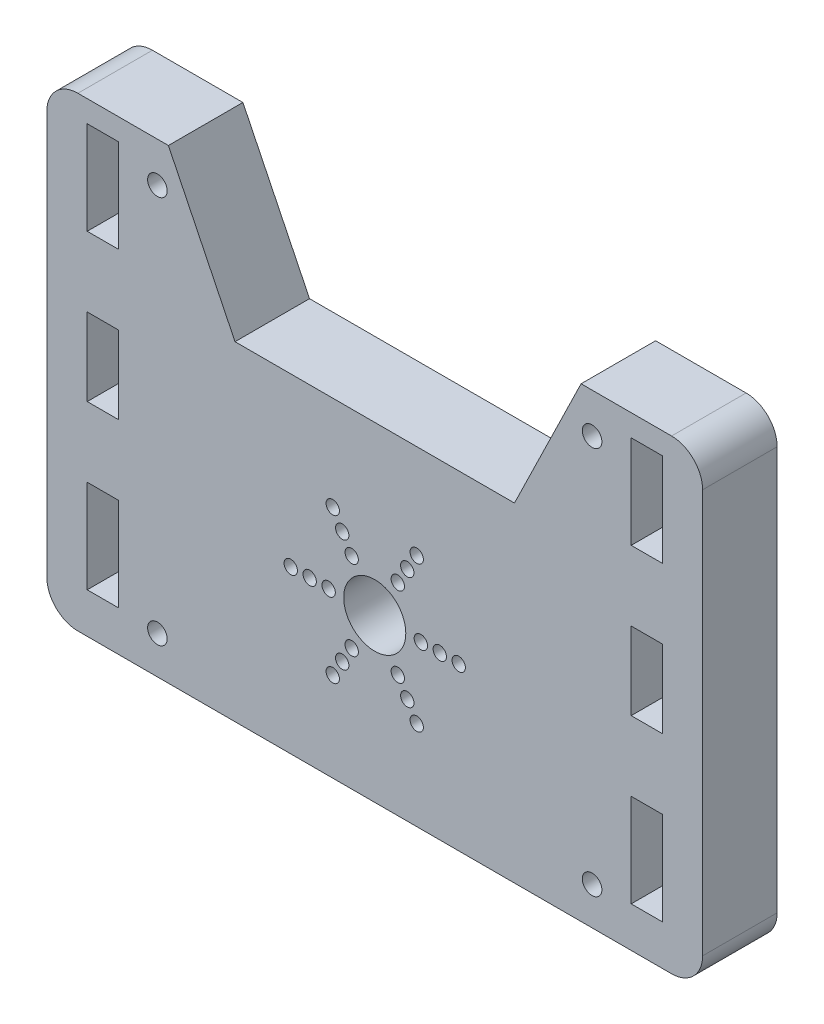
SolidWorks part; units mm, degrees
ref_plane "前视基准面" through (0, 0, 0) normal (0, 0, 1) x (1, 0, 0)
ref_plane "上视基准面" through (0, 0, 0) normal (0, 1, 0) x (1, 0, 0)
ref_plane "右视基准面" through (0, 0, 0) normal (1, 0, 0) x (0, 0, -1)
other "Configuration Table"
sketch "草图1" plane through (0, 0, 0) normal (0, 0, 1) x (1, 0, 0)
  line L0 (0, 52.9649) -> (0, -55.4114) construction
  line L1 (-89.1236, 0) -> (105.0799, 0) construction
  line L2 (-33.1441, 37.4747) -> (-22.414, 15.4747)
  line L3 (-47.714, 37.4747) -> (-33.1441, 37.4747)
  line L4 (-52.714, 32.4747) -> (-52.714, -32.5253)
  line L5 (-47.714, -37.5253) -> (47.886, -37.5253)
  line L6 (52.886, 32.4747) -> (52.886, -32.5253)
  line L7 (-22.414, 15.4747) -> (22.586, 15.4747)
  line L8 (22.586, 15.4747) -> (33.3161, 37.4747)
  line L9 (-41.214, -31.0253) -> (-46.214, -31.0253)
  line L10 (41.386, -16.0253) -> (46.386, -16.0253)
  line L11 (41.386, -16.0253) -> (41.386, -31.0253)
  line L12 (41.386, -31.0253) -> (46.386, -31.0253)
  line L13 (46.386, -16.0253) -> (46.386, -31.0253)
  line L14 (41.386, 7.7247) -> (46.386, 7.7247)
  line L15 (41.386, 7.7247) -> (41.386, -4.7753)
  line L16 (41.386, -4.7753) -> (46.386, -4.7753)
  line L17 (46.386, 7.7247) -> (46.386, -4.7753)
  line L18 (41.386, 33.9747) -> (46.386, 33.9747)
  line L19 (41.386, 33.9747) -> (41.386, 18.9747)
  line L20 (41.386, 18.9747) -> (46.386, 18.9747)
  line L21 (46.386, 33.9747) -> (46.386, 18.9747)
  line L22 (-46.214, -16.0253) -> (-46.214, -31.0253)
  line L23 (-41.214, -16.0253) -> (-46.214, -16.0253)
  line L24 (-41.214, -16.0253) -> (-41.214, -31.0253)
  line L25 (-41.214, -4.7753) -> (-46.214, -4.7753)
  line L26 (-46.214, 7.7247) -> (-46.214, -4.7753)
  line L27 (-41.214, 7.7247) -> (-46.214, 7.7247)
  line L28 (-41.214, 7.7247) -> (-41.214, -4.7753)
  line L29 (-41.214, 18.9747) -> (-46.214, 18.9747)
  line L30 (-46.214, 33.9747) -> (-46.214, 18.9747)
  line L31 (-41.214, 33.9747) -> (-46.214, 33.9747)
  line L32 (-41.214, 33.9747) -> (-41.214, 18.9747)
  line L33 (33.3161, 37.4747) -> (47.886, 37.4747)
  circle A0 centre (35.086, 31.0553) radius 1.575
  circle A1 centre (35.086, -31.4447) radius 1.575
  circle A2 centre (0.086, -11.4447) radius 13.525 construction
  circle A3 centre (0.086, -11.4447) radius 5
  circle A4 centre (7.511, -11.4447) radius 1.075
  circle A5 centre (10.561, -11.4447) radius 1.075
  circle A6 centre (13.611, -11.4447) radius 1.075
  circle A7 centre (5.3235, -20.5163) radius 1.075
  circle A8 centre (3.7985, -17.8749) radius 1.075
  circle A9 centre (6.8485, -23.1577) radius 1.075
  circle A10 centre (-5.1515, -20.5163) radius 1.075
  circle A11 centre (-3.6265, -17.8749) radius 1.075
  circle A12 centre (-6.6765, -23.1577) radius 1.075
  circle A13 centre (-10.389, -11.4447) radius 1.075
  circle A14 centre (-7.339, -11.4447) radius 1.075
  circle A15 centre (-13.439, -11.4447) radius 1.075
  circle A16 centre (-5.1515, -2.3731) radius 1.075
  circle A17 centre (-3.6265, -5.0145) radius 1.075
  circle A18 centre (-6.6765, 0.2683) radius 1.075
  circle A19 centre (5.3235, -2.3731) radius 1.075
  circle A20 centre (3.7985, -5.0145) radius 1.075
  circle A21 centre (6.8485, 0.2683) radius 1.075
  circle A22 centre (-34.914, 31.0553) radius 1.575
  circle A23 centre (-34.914, -31.4447) radius 1.575
  arc A24 (47.886, -37.5253) -> (52.886, -32.5253) centre (47.886, -32.5253) ccw
  arc A25 (-52.714, -32.5253) -> (-47.714, -37.5253) centre (-47.714, -32.5253) ccw
  arc A26 (47.886, 37.4747) -> (52.886, 32.4747) centre (47.886, 32.4747) cw
  arc A27 (-47.714, 37.4747) -> (-52.714, 32.4747) centre (-47.714, 32.4747) ccw
  dimension "D12" = 3.15
  dimension "D13" = 27.05
  dimension "D14" = 10
  dimension "D17" = 2.15
  dimension "D18" = 5
  dimension "D1" = 45
  dimension "D2" = 53
  dimension "D3" = 64
  dimension "D4" = 5
  dimension "D5" = 15
  dimension "D6" = 12.5
  dimension "D7" = 15
  dimension "D8" = 3.5
  dimension "D9" = 11.25
  dimension "D10" = 11.25
  dimension "D11" = 6.5
  dimension "D15" = 3.05
  dimension "D16" = 3.05
extrude "凸台-拉伸1" add sketch "草图1" along normal blind 12
